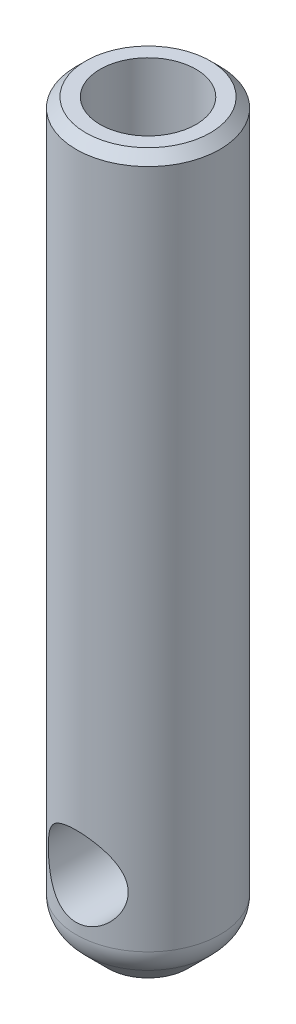
from build123d import *

# Parameters (mm, degrees)
SKETCH_1_R              = 22.5
EXTRUDE_1_DEPTH         = 250
SKETCH_2_R              = 15
CUT_EXTRUDE_1_DEPTH     = 200
CUT_EXTRUDE2_DEPTH      = 210
CUT_EXTRUDE2_DEPTH_BACK = 210
SKETCH_3_R              = 12.5
SKETCH_4_R              = 53.120468805
CUT_EXTRUDE3_DEPTH      = 20
CHAMFER1_SIZE           = 10
CHAMFER2_SIZE           = 3
FILLET1_R               = 10


with BuildPart() as part:
    # 草图1 → 凸台-拉伸1 (new body)
    with BuildSketch(Plane(origin=(0, 0, 0), x_dir=(1, 0, 0), z_dir=(0, 1, 0))):
        with Locations(Location((0, 0, 0), (0, 0, 270))):
            Circle(SKETCH_1_R)
    extrude(amount=EXTRUDE_1_DEPTH)

    # 草图2 → 切除-拉伸1 (cut)
    with BuildSketch(Plane(origin=(0, 250, 0), x_dir=(1, 0, 0), z_dir=(0, 1, 0))):
        with Locations(Location((0, 0, 0), (0, 0, 270))):
            Circle(SKETCH_2_R)
    extrude(amount=-CUT_EXTRUDE_1_DEPTH, mode=Mode.SUBTRACT)

    # 草图3 → Cut-Extrude2 (cut, two sides: drawn at the far end of the back side and taken through both)
    with BuildSketch(Plane.XY.offset(-CUT_EXTRUDE2_DEPTH_BACK)):
        with Locations(Location((0, 30, 0), (0, 0, 90))):
            Circle(SKETCH_3_R)
    extrude(amount=CUT_EXTRUDE2_DEPTH + CUT_EXTRUDE2_DEPTH_BACK, mode=Mode.SUBTRACT)

    # 草图4 → Cut-Extrude3 (cut)
    with BuildSketch(Plane(origin=(0, 250, 0), x_dir=(1, 0, 0), z_dir=(0, 1, 0))):
        Circle(SKETCH_4_R)
    extrude(amount=-CUT_EXTRUDE3_DEPTH, mode=Mode.SUBTRACT)

    # Chamfer1
    chamfer1_edges = [part.edges().sort_by_distance(p)[0] for p in [
        (0, 0, -22.5),
    ]]
    chamfer(chamfer1_edges, length=CHAMFER1_SIZE)

    # Chamfer2
    chamfer2_edges = [part.edges().sort_by_distance(p)[0] for p in [
        (0, 230, -22.5),
    ]]
    chamfer(chamfer2_edges, length=CHAMFER2_SIZE)

    # Fillet1
    fillet1_edges = [part.edges().sort_by_distance(p)[0] for p in [
        (0, 10, -22.5),
    ]]
    fillet(fillet1_edges, radius=FILLET1_R)


solid = part.part
